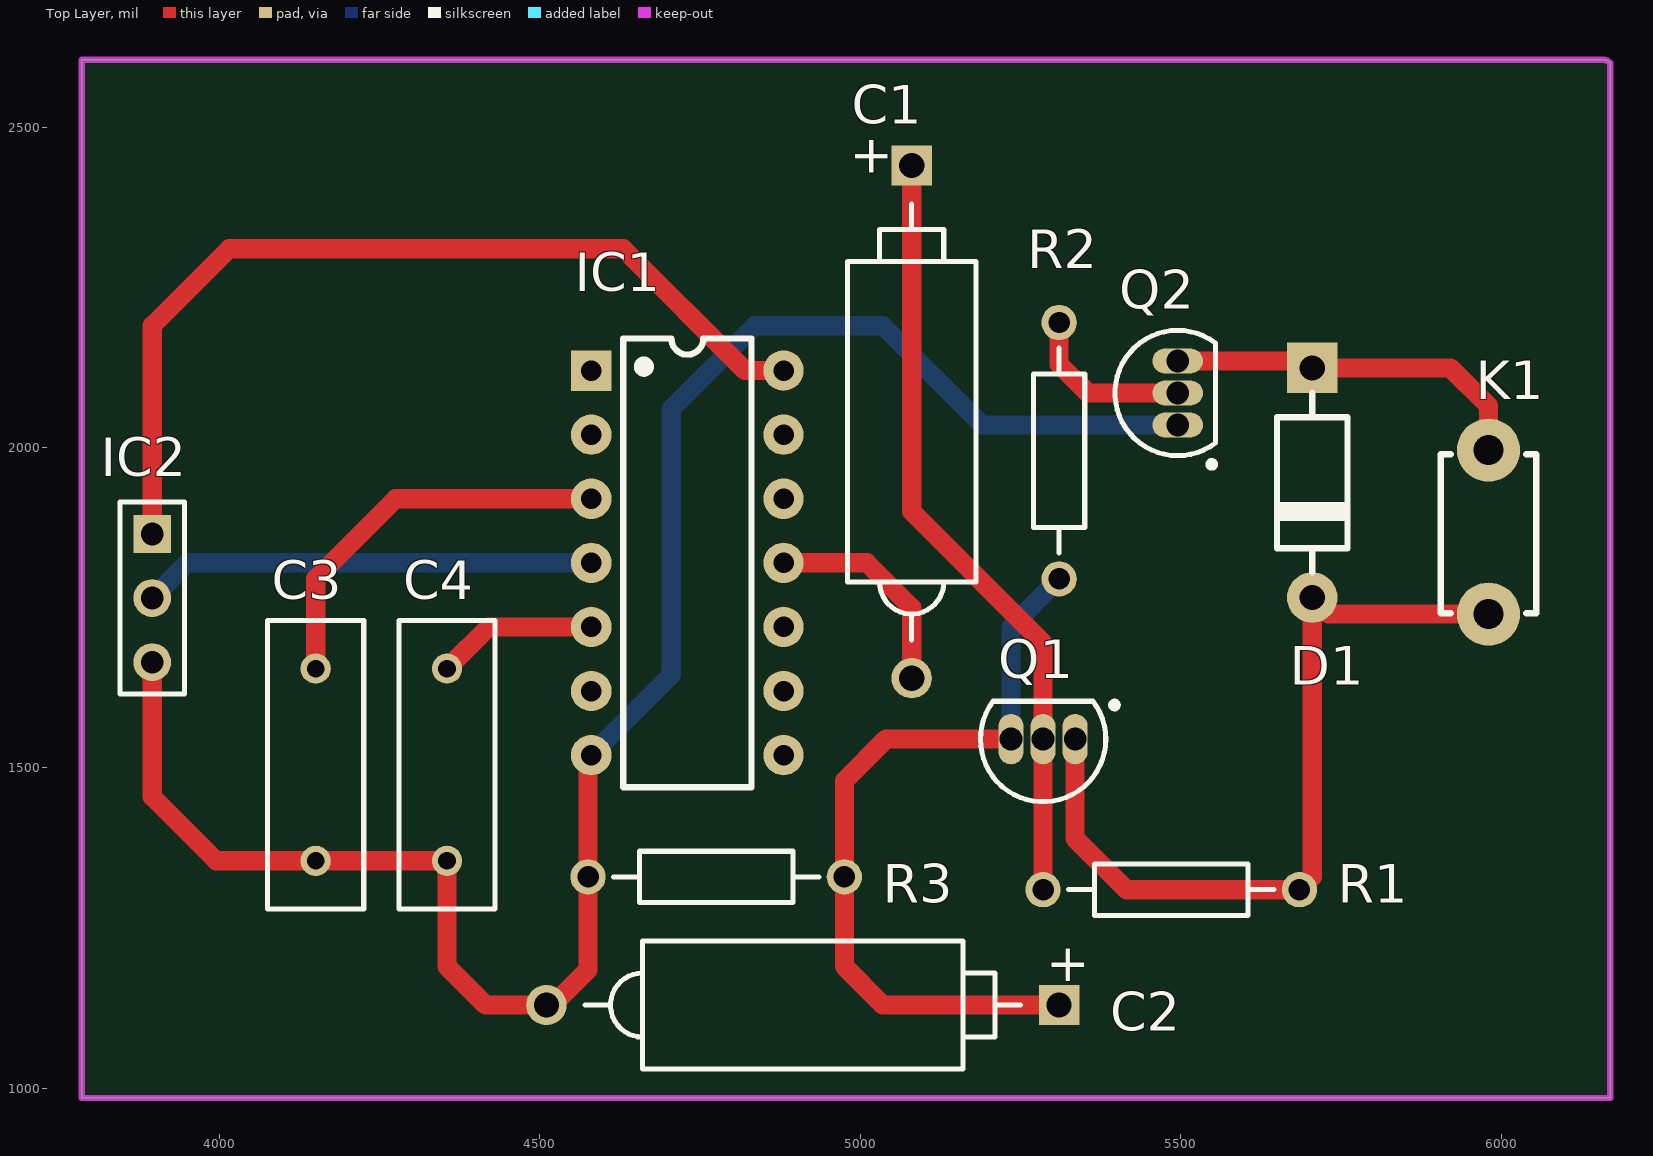
[diagram p0: Top Layer view]
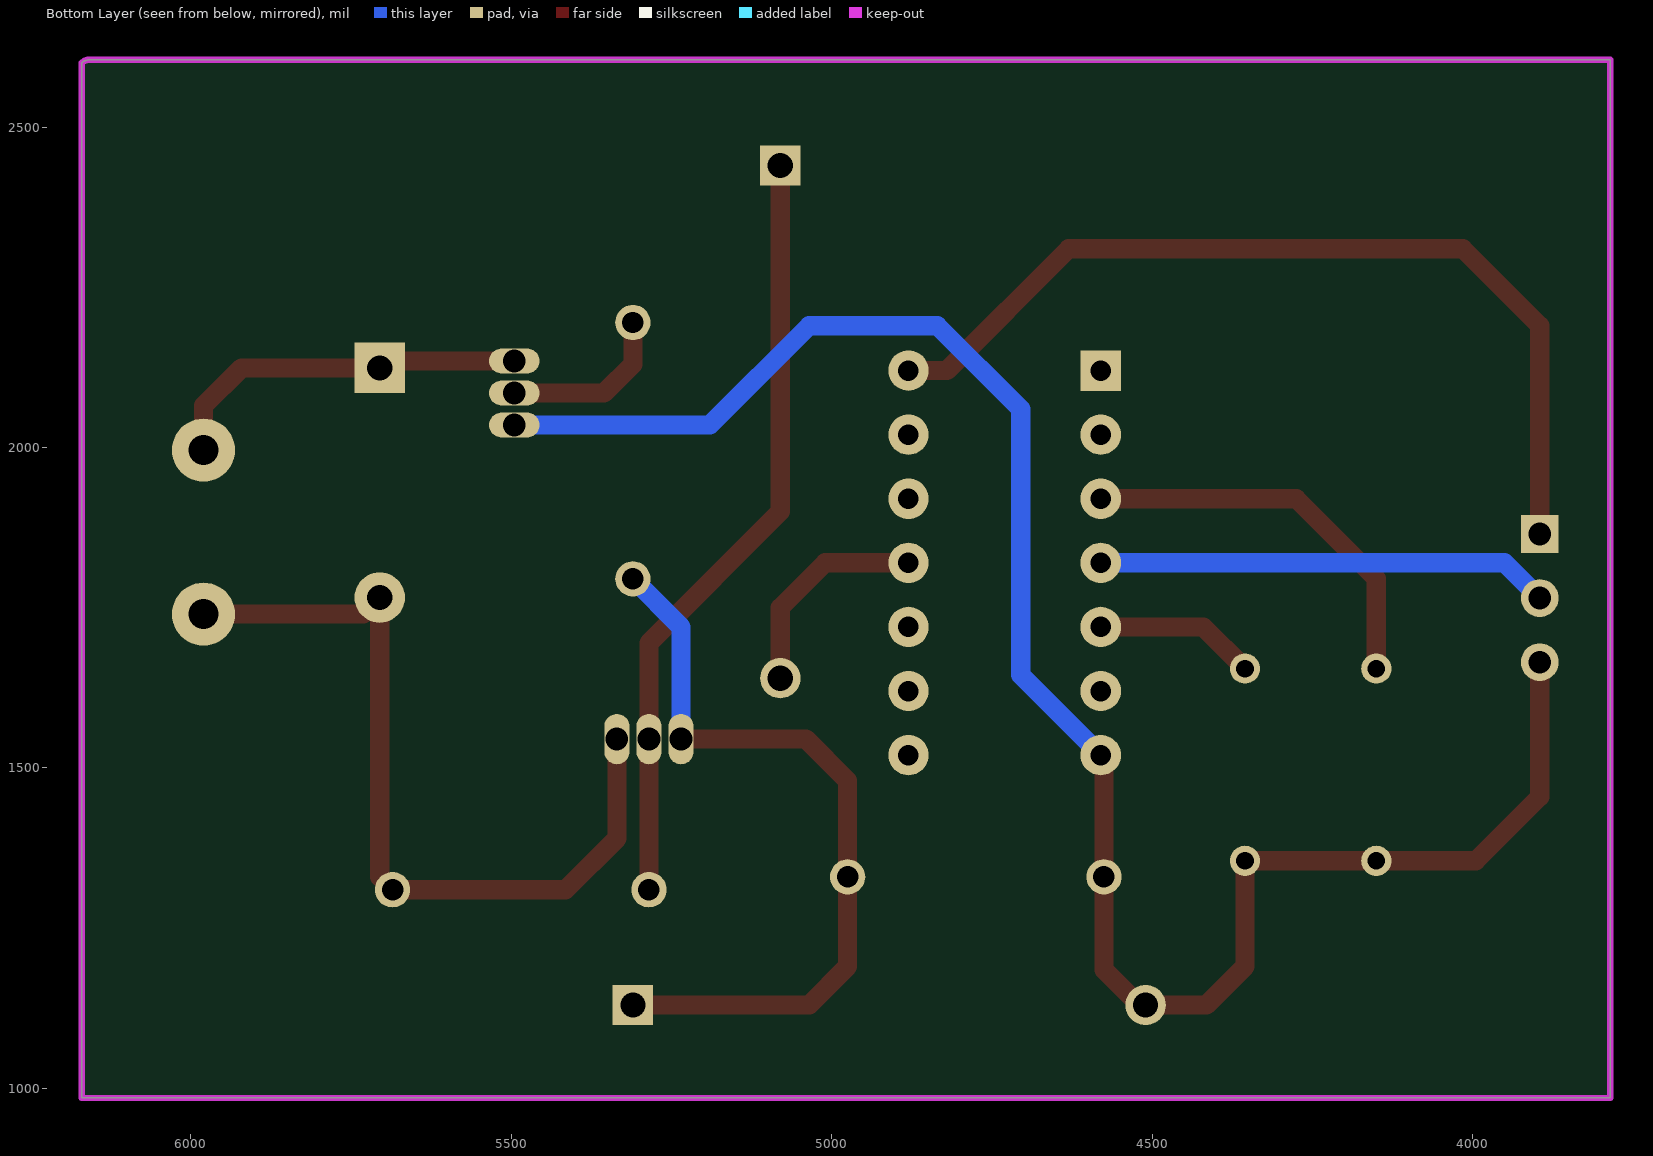
[diagram p1: Bottom Layer view, seen from below]
# Altium PCB MISC80621.PcbDoc
Units mil, origin at the board's own origin, x right, y up, seen from the top; angles counter-clockwise.
Board outline 2385 x 1620 mil, 2 copper layers (Top Layer, Bottom Layer); 13 components, 11 nets, 41 pads, 0 vias.

## Layer stack, top to bottom (the 12.6 mil dielectric is the usual default, probably not edited)
Top Solder: solder mask 0.4, Solder Resist, Dk 3.5
Top Layer: signal copper 1.4
Dielectric 1: dielectric 12.6, FR-4, Dk 4.8
Bottom Layer: signal copper 1.4
Bottom Solder: solder mask 0.4, Solder Resist, Dk 3.5

## Board outline
3785,985 6170,985 6170,2600 ccw(c6157.93,2587.93) 6157.93,2605 3785,2605

## Design rules (kind name [scope] priority, off if disabled: settings)
Clearance [All] p1: gap=10
MinimumSolderMaskSliver [All] p1: minsoldermaskwidth=0
PolygonConnect [All] p1: connectstyle=Relief reliefconductorwidth=10 reliefentries=4 polygonreliefangle="90 Angle" airgapwidth=10
RoutingVias [All] p1: holewidth=28 width=50 viastyle="Through Hole" minholewidth=28 minwidth=50 maxholewidth=28 maxwidth=50
SilkToSilkClearance [All] p1: silktosilkclearance=0
SilkToSolderMaskClearance [IsPad] p1: minsilkscreentomaskgap=0 clearancetoexposedcopper=TRUE
SolderMaskExpansion [All] p1: expansion=4
Width [All] p1: maxlimit=30 minlimit=10 preferedwidth=10
27 further rules are at their usual default settings.

## Components (designator, comment, footprint, x,y, rotation, side; value= is the part's Value field where it differs from the comment)
C1 "1UF" POLAR0.8 5080,2040 r90 top
C2 "100UF" POLAR0.8 4910,1130 r0 top
C3 "0.022UF" RAD-0.3 4150,1505 r90 top
C4 "3300PF" RAD-0.3 4355,1505 r90 top
D1 "1N4001" DO-41 5705,1945 r270 top
IC1 "LC9305" DIP14 4580,2120 r0 top
IC2 "BA5302" HDR1X3 3895,1865 r270 top
K1 "KEY" DIP-3X6X4.3 5980,1995.91 r270 top
Q1 "9012" TO-92A 5285,1545 r90 top
Q2 "8050" TO-92A 5495,2085 r0 top
R1 "10K" AXIAL-0.4 5485,1310 r0 top
R2 "510" AXIAL-0.4 5310,1995 r270 top
R3 "100K" AXIAL-0.4 4775,1330 r0 top

## Footprints (in the part's own frame and the unit in brackets; to place one, negate y for a bottom-side part, rotate by r counter-clockwise, add the part's x,y. Pads: shape width x height; smd on the part's side, far side on the other; paste and mask are expansions set on the pad)
AXIAL-0.4 [mm] "Axial Device, Thru-Hole; 2 Leads; 0.4 in Pin Spacing"
  round 1.4 hole 0.85: 1(-5.08,0) 2(5.08,0)
  silkscreen extent -4.06,-1.02 4.06,1.02
DIP14 [mm]
  rect 1.6x1.6 hole 0.813: 1(0,0)
  round 1.6 hole 0.813: 2(0,-2.54) 3(0,-5.08) 4(0,-7.62) 5(0,-10.16) 6(0,-12.7) 7(0,-15.24) 8(7.62,-15.24) 9(7.62,-12.7) 10(7.62,-10.16) 11(7.62,-7.62) 12(7.62,-5.08) 13(7.62,-2.54) 14(7.62,0)
  silkscreen extent 1.27,-16.51 6.35,1.27, body extent -0.25,-17.62 7.62,2.38, height 5.1
DIP-3X6X4.3 [mm]
  round 2.5 hole 1.2: 1(0,0) 3(6.5,0)
  silkscreen extent 0.16,-1.9 6.46,1.9, body extent -0.64,-1.75 7.19,1.75, height 4.31
DO-41 [mm] "2.6*9.1mm(直径，脚距）"
  rect 2x2 hole 1: 1(-4.55,0)
  round 2 hole 1: 2(4.55,0)
  silkscreen extent -3.56,-1.4 3.56,1.4, body extent -4.92,-1.29 4.98,1.31, height 2.65
HDR1X3 [mm] "Connector; Header; 3 Position"
  rect 1.5x1.5 hole 0.9: 1(0,0)
  round 1.5 hole 0.9: 2(2.54,0) 3(5.08,0)
  silkscreen extent -1.27,-1.27 6.35,1.27
POLAR0.8 [mm] "Polarized Capacitor; 2 Leads"
  rect 1.6x1.6 hole 1: 1(10.16,0)
  round 1.6 hole 1: 2(-10.16,0)
  silkscreen extent -8.64,-2.54 8.64,2.54
RAD-0.3 [mm] "Radial Cap, Thru-Hole; 2 Leads; 0.3 in Pin Spacing"
  round 1.2 hole 0.7: 1(-3.81,0) 2(3.81,0)
  silkscreen extent -5.71,-1.91 5.71,1.91
TO-92A [mm] "TO, Flat Index; 3 In-Line, Axial Leads; Body Dia. 4.5mm; Leads 0.51 x 0.48 mm (max)"
  oval 2x1 hole 0.9: 1(0,-1.27) 2(0,0) 3(0,1.27)
  silkscreen extent -2.48,-2.96 1.5,2.48, body extent -2.48,-2.5 1.5,2.5, height 6.86

## Part data
C1 C2: library part "Cap Pol2", "Polarized Capacitor (Axial)"
C3 C4: library part Cap, "Capacitor"
D1: library part 1N4007, "Rectifier diode"
Q1: library part 2N3906, "PNP General Purpose Amplifier"
Q2: library part 2N3904, "NPN General Purpose Amplifier"
R1 R2 R3: library part Res2, "Resistor"

## Nets (pads, with @x,y where several pads share a name; then routed paths per layer and width w, separated by ;. In a path a pad name is that pad's centre, name@x,y a point inside that pad or via, vN(x,y) a via of type N, cw(c..) or ccw(c..) an arc to the next point about the centre after c; other vN are vias at no path point)
+5V: IC1.14 IC2.1 | length 1438.4
  Top Layer w30: IC2.1 3895,2190 4015,2310 4630,2310 4820,2120 IC1.14
GND: C2.2 C3.1 C4.1 IC1.7 IC2.3 Q2.1 R3.1 | length 2981
  Top Layer w30: IC2.3 3895,1455 3995,1355 C3.1 C4.1 4355,1190 4415,1130 C2.2 4520,1130 4575,1185 R3.1 4575,1515 IC1.7
  Bottom Layer w30: IC1.7 4705,1645 4705,2060 4835,2190 5035,2190 5190,2035 Q2.1
NetC1_1: C1.1 Q1.2 R1.1 | length 1214.9
  Top Layer w30: C1.1 5080,1900 5285,1695 Q1.2 R1.1
NetC1_2: C1.2 IC1.11 | length 339
  Top Layer w30: IC1.11 5010,1820 5080,1750 C1.2
NetC2_1: C2.1 Q1.3 R2.2 R3.2 | length 1217.8
  Top Layer w30: Q1.3 5040,1545 4975,1480 R3.2 4975,1190 5035,1130 C2.1
  Bottom Layer w30: Q1.3 5235,1720 R2.2
NetC3_2: C3.2 IC1.3 | length 621.8
  Top Layer w30: C3.2 4150,1795 4275,1920 IC1.3
NetC4_2: C4.2 IC1.5 | length 251.9
  Top Layer w30: C4.2 4420,1720 IC1.5
NetD1_1: D1.1 K1.1 Q2.3 | length 583.1
  Top Layer w30: Q2.3 5694.13,2135 D1.1 5920.87,2124.13 5980,2065 K1.1
NetIC1_4: IC1.4 IC2.2 | length 707.8
  Bottom Layer w30: IC2.2 3950,1820 IC1.4
NetQ2_2: Q2.2 R2.1 | length 268.6
  Top Layer w30: R2.1 5310,2130 5355,2085 Q2.2
U: D1.2 K1.3 Q1.1 R1.2 | length 1288
  Top Layer w30: Q1.1 5335,1390 5415,1310 R1.2 5705,1330 D1.2 5730.87,1740 K1.3
pads on no net: IC1.1 IC1.2 IC1.6 IC1.8 IC1.9 IC1.10 IC1.12 IC1.13

## Keep-outs
Keep-Out Layer:
  the board outline again, w10